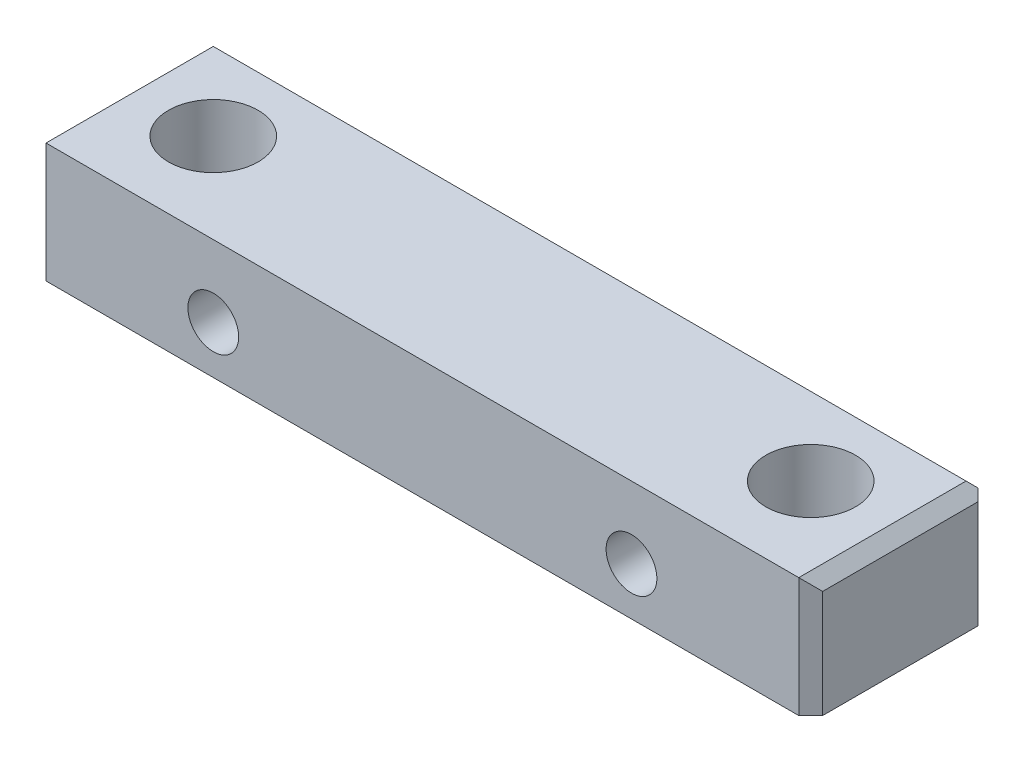
SolidWorks part; units mm, degrees
ref_plane "前视基准面" through (0, 0, 0) normal (0, 0, 1) x (1, 0, 0)
ref_plane "上视基准面" through (0, 0, 0) normal (0, 1, 0) x (1, 0, 0)
ref_plane "右视基准面" through (0, 0, 0) normal (1, 0, 0) x (0, 0, -1)
sketch "草图1" plane through (0, 0, 0) normal (0, 0, 1) x (1, 0, 0)
  line L1 (-65, 10) -> (65, 10)
  line L2 (-65, 10) -> (-65, -10)
  line L3 (-65, -10) -> (65, -10)
  line L4 (65, 10) -> (65, -10)
  line L5 (-65, 10) -> (65, -10) construction
  line L6 (-65, -10) -> (65, 10) construction
  point P0 (0, 0)
  dimension "D1" = 20
  dimension "D2" = 130
extrude "凸台-拉伸1" add sketch "草图1" along normal blind 30
hole_wizard "打孔尺寸(%根据)内六角圆柱头螺钉的类型1" positions "草图2" profile "草图3" counterbore size "M8" standard "GB" end condition through all
sketch "草图2" plane through (0, 10, 0) normal (0, 1, 0) x (1, 0, 0)
  line L0 (0, 0) -> (0, -40.624) construction
  line L2 (65, -15) -> (9.9649, -15) construction
  line L3 (65, -30) -> (65, 0) construction
  point P0 (-50, -15)
  point P2 (50, -15)
  dimension "D1" = 100
sketch "草图3" plane through (-50, 10, 15) normal (1, 0, 0) x (0, 0, 1)
  line L0 (0, 0) -> (0, 20)
  line L1 (0, 20) -> (4.5, 20)
  line L3 (4.5, 20) -> (4.5, 15)
  line L4 (4.5, 15) -> (7.5, 15)
  line L5 (7.5, 15) -> (7.5, 0)
  line L7 (7.5, 0) -> (0, 0)
  line L11 (0, -6.35) -> (0, 107.95) construction
  dimension "通孔孔直径" = 9
  dimension "通孔孔深度" = 20
  dimension "柱形沉头孔直径" = 15
  dimension "柱形沉头孔深度" = 15
hole_wizard "M10 螺纹孔1" positions "草图4" profile "草图5" tap size "M10" standard "GB" end condition through all
sketch "草图4" plane through (0, 0, 30) normal (0, 0, 1) x (1, 0, 0)
  line L0 (0, 41.3926) -> (0, 0) construction
  line L2 (-65, -10) -> (65, -10) construction
  point P0 (-35, -2)
  point P2 (35, -2)
  dimension "D1" = 70
  dimension "D2" = 8
sketch "草图5" plane through (-35, -2, 30) normal (1, 0, 0) x (0, -1, 0)
  line L0 (0, 0) -> (0, 30)
  line L1 (0, 30) -> (4.25, 30)
  line L2 (4.25, 30) -> (4.25, 0)
  line L5 (4.25, 0) -> (0, 0)
  line L11 (0, -6.35) -> (0, 107.95) construction
  dimension "通孔螺纹孔钻头直径" = 8.5
  dimension "通孔螺纹孔钻头深度" = 30
cosmetic thread "孔螺蚊线1" parameters "D2"=10
cosmetic thread "孔螺蚊线2" parameters "D2"=10
chamfer "倒角1" distance 2 angle 45 6 edges at (-65, 0, 0) (-65, 10, 15) (-65, 0, 30) (65, 0, 0) (65, 10, 15) (65, 0, 30)
chamfer "倒角2" distance 2 angle 45 1 edges at (0, 10, 0)
